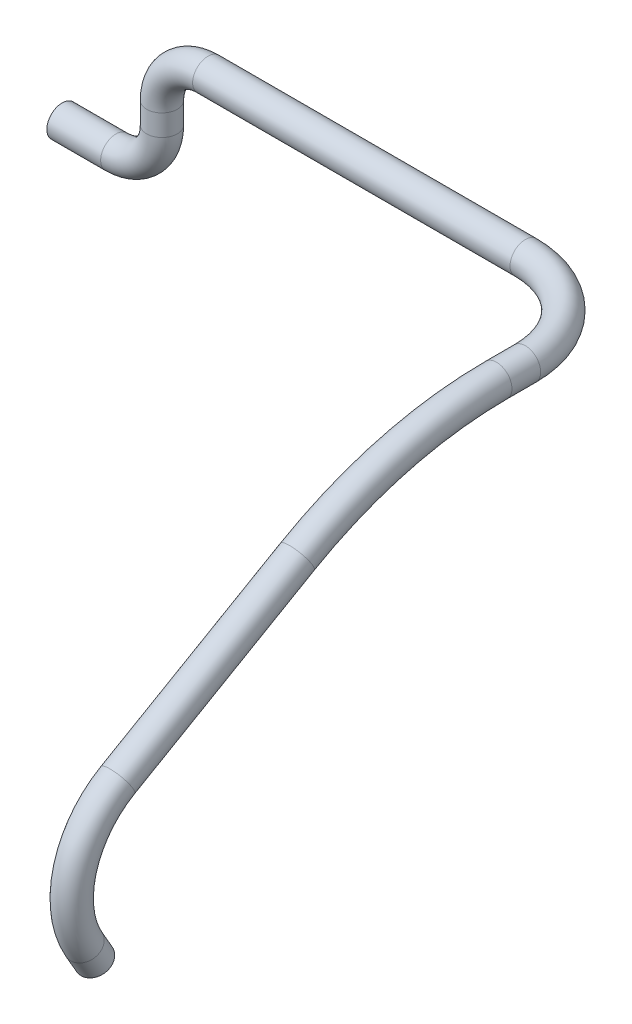
from build123d import *

# Parameters (mm, degrees)
SKETCH1_R = 2


with BuildPart() as part:
    # Sweep1: sweep along a curve in space
    with BuildLine() as sweep1_path:
        Line((-50.19826571, 33.779851644, 68.304462045), (-50.190924205, 36.164146317, 69.680554329))
        ThreePointArc((-50.190924205, 36.164146317, 69.680554329), (-50.168295566, 45.270129978, 70.877966766), (-50.158922477, 52.555749547, 65.285748364))
        Line((-50.158922477, 52.555749547, 65.285748364), (-50.158922477, 66.080807741, 41.85147393))
        ThreePointArc((-50.158922477, 73.043553961, 15.8582869), (-50.158922477, 71.272714796, 29.313077932), (-50.158922477, 66.080807741, 41.85147393))
        Line((-50.158922477, 73.043553961, 15.8582869), (-50.158922477, 73.043553961, 12.109558404))
        ThreePointArc((-62.158922477, 73.043553961, 0.109558404), (-53.673641103, 73.043553961, 3.62427703), (-50.158922477, 73.043553961, 12.109558404))
        Line((-103.577768148, 73.043553961, 0.109558404), (-62.158922477, 73.043553961, 0.109558404))
        ThreePointArc((-103.577768148, 73.043553961, 0.109558404), (-107.820408835, 71.286194648, 0.109558404), (-109.577768148, 67.043553961, 0.109558404))
        Line((-109.577768148, 64.263552475, 0.109558404), (-109.577768148, 67.043553961, 0.109558404))
        ThreePointArc((-109.577768148, 64.263552475, 0.109558404), (-111.335127461, 60.020911788, 0.109558404), (-115.577768148, 58.263552475, 0.109558404))
        Line((-122.59826571, 58.263552475, 0.109558404), (-115.577768148, 58.263552475, 0.109558404))
    # Sketch1 → Sweep1 (sweep)
    with BuildSketch(Plane(origin=(-122.59826571, 0, 0), x_dir=(0, 0, -1), z_dir=(1, 0, 0))):
        with Locations((-0.109558404, 58.263552475)):
            Circle(SKETCH1_R)
    sweep(path=sweep1_path.line)


solid = part.part
